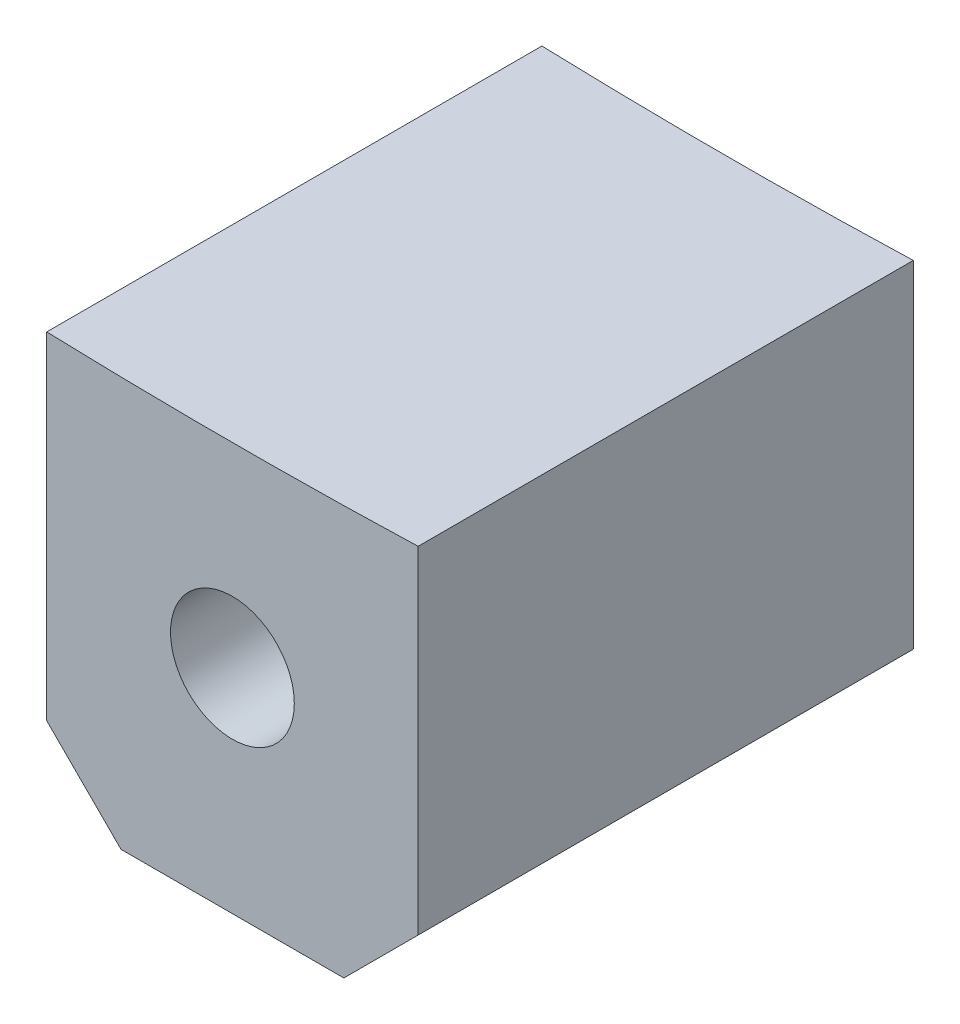
from build123d import *

# Parameters (mm, degrees)
BOSS_EXTRUDE1_DEPTH = 20
CHAMFER1_SIZE       = 3
M6_TAPPED_HOLE1_D   = 5


with BuildPart() as part:
    # Sketch1 → Boss-Extrude1 (new body)
    with BuildSketch(Plane.XY):
        with BuildLine():
            Line((-7.5, -231.178372691), (-7.5, -247.778372691))
            Line((-7.5, -247.778372691), (7.5, -247.778372691))
            Line((7.5, -247.778372691), (7.5, -231.178372691))
            ThreePointArc((7.5, -231.178372691), (0, -231.3), (-7.5, -231.178372691))
        make_face()
    extrude(amount=BOSS_EXTRUDE1_DEPTH)

    # Chamfer1
    chamfer1_edges = [part.edges().sort_by_distance(p)[0] for p in [
        (7.5, -247.778372691, 10),
        (-7.5, -247.778372691, 10),
    ]]
    chamfer(chamfer1_edges, length=CHAMFER1_SIZE)

    # M6 Tapped Hole1 (through all)
    with Locations(Plane.XY.offset(20)):
        with Locations((0, -239.178372691)):
            Hole(M6_TAPPED_HOLE1_D / 2)


solid = part.part
